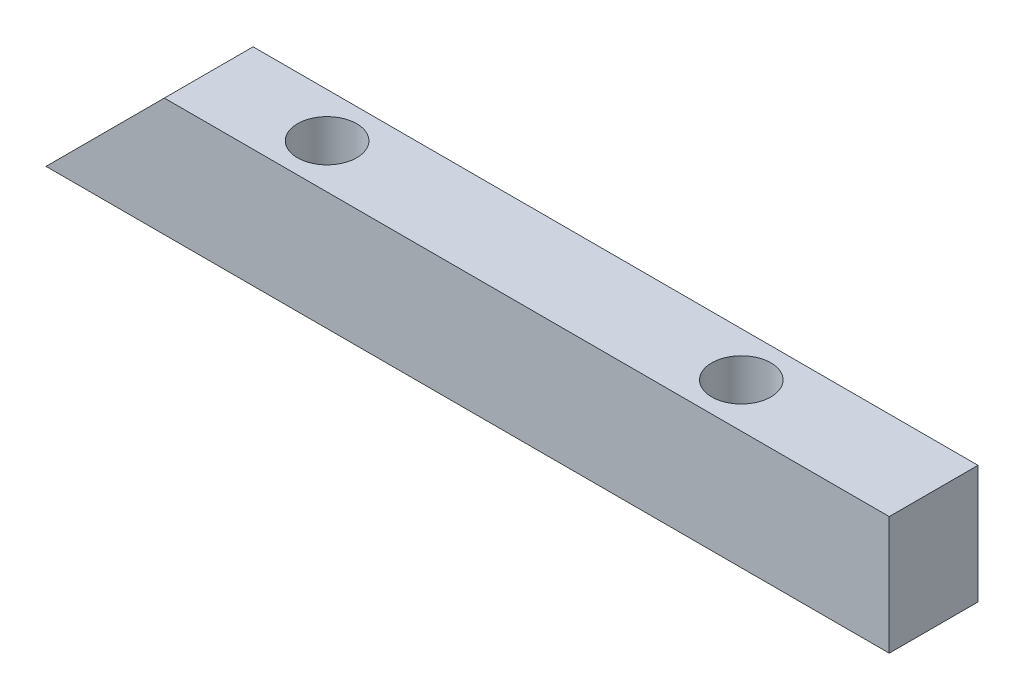
SolidWorks part; units mm, degrees
ref_plane "前视基准面" through (0, 0, 0) normal (0, 0, 1) x (1, 0, 0)
ref_plane "上视基准面" through (0, 0, 0) normal (0, 1, 0) x (1, 0, 0)
ref_plane "右视基准面" through (0, 0, 0) normal (1, 0, 0) x (0, 0, -1)
sketch "草图1" plane through (0, 0, 0) normal (0, 1, 0) x (1, 0, 0)
  line L1 (-135, -15) -> (135, -15)
  line L2 (-135, -15) -> (-135, 15)
  line L3 (-135, 15) -> (135, 15)
  line L4 (135, -15) -> (135, 15)
  line L5 (-135, -15) -> (135, 15) construction
  line L6 (-135, 15) -> (135, -15) construction
  point P0 (0, 0)
  dimension "D1" = 270
  dimension "D2" = 30
extrude "凸台-拉伸1" add sketch "草图1" along normal blind 40
sketch "草图2" plane through (0, 40, 0) normal (0, 1, 0) x (1, 0, 0)
  line L1 (0, 0) -> (0, 40) construction
  circle A0 centre (70, 0) radius 10
  circle A1 centre (-70, 0) radius 10
  dimension "D1" = 20
  dimension "D2" = 140
  dimension "D3" = 40
extrude "切除-拉伸2" cut sketch "草图2" against normal blind 30
sketch "草图3" plane through (-135, 0, 0) normal (-1, 0, 0) x (0, 0, 1)
  line L4 (-15, 0) -> (15, 0)
  line L5 (15, 0) -> (15, 40)
  line L6 (15, 40) -> (-15, 40)
  line L7 (-15, 40) -> (-15, 0)
  line L8 (-15, 0) -> (15, 0)
  line L9 (15, 0) -> (15, 40)
  line L10 (15, 40) -> (-15, 40)
  line L11 (-15, 40) -> (-15, 0)
  dimension "D1" = 0
extrude "凸台-拉伸2" add sketch "草图3" along normal blind 15
sketch "草图4" plane through (0, 0, 15) normal (0, 0, 1) x (1, 0, 0)
  line L0 (-150, 0) -> (-110, 40)
  line L1 (-150, 40) -> (135, 40) construction
  line L2 (-150, 0) -> (-150, 40) construction
  line L3 (-150, 0) -> (-150, 40)
  line L4 (-150, 40) -> (-110, 40)
  dimension "D1" = 45
extrude "切除-拉伸3" cut sketch "草图4" against normal through all
